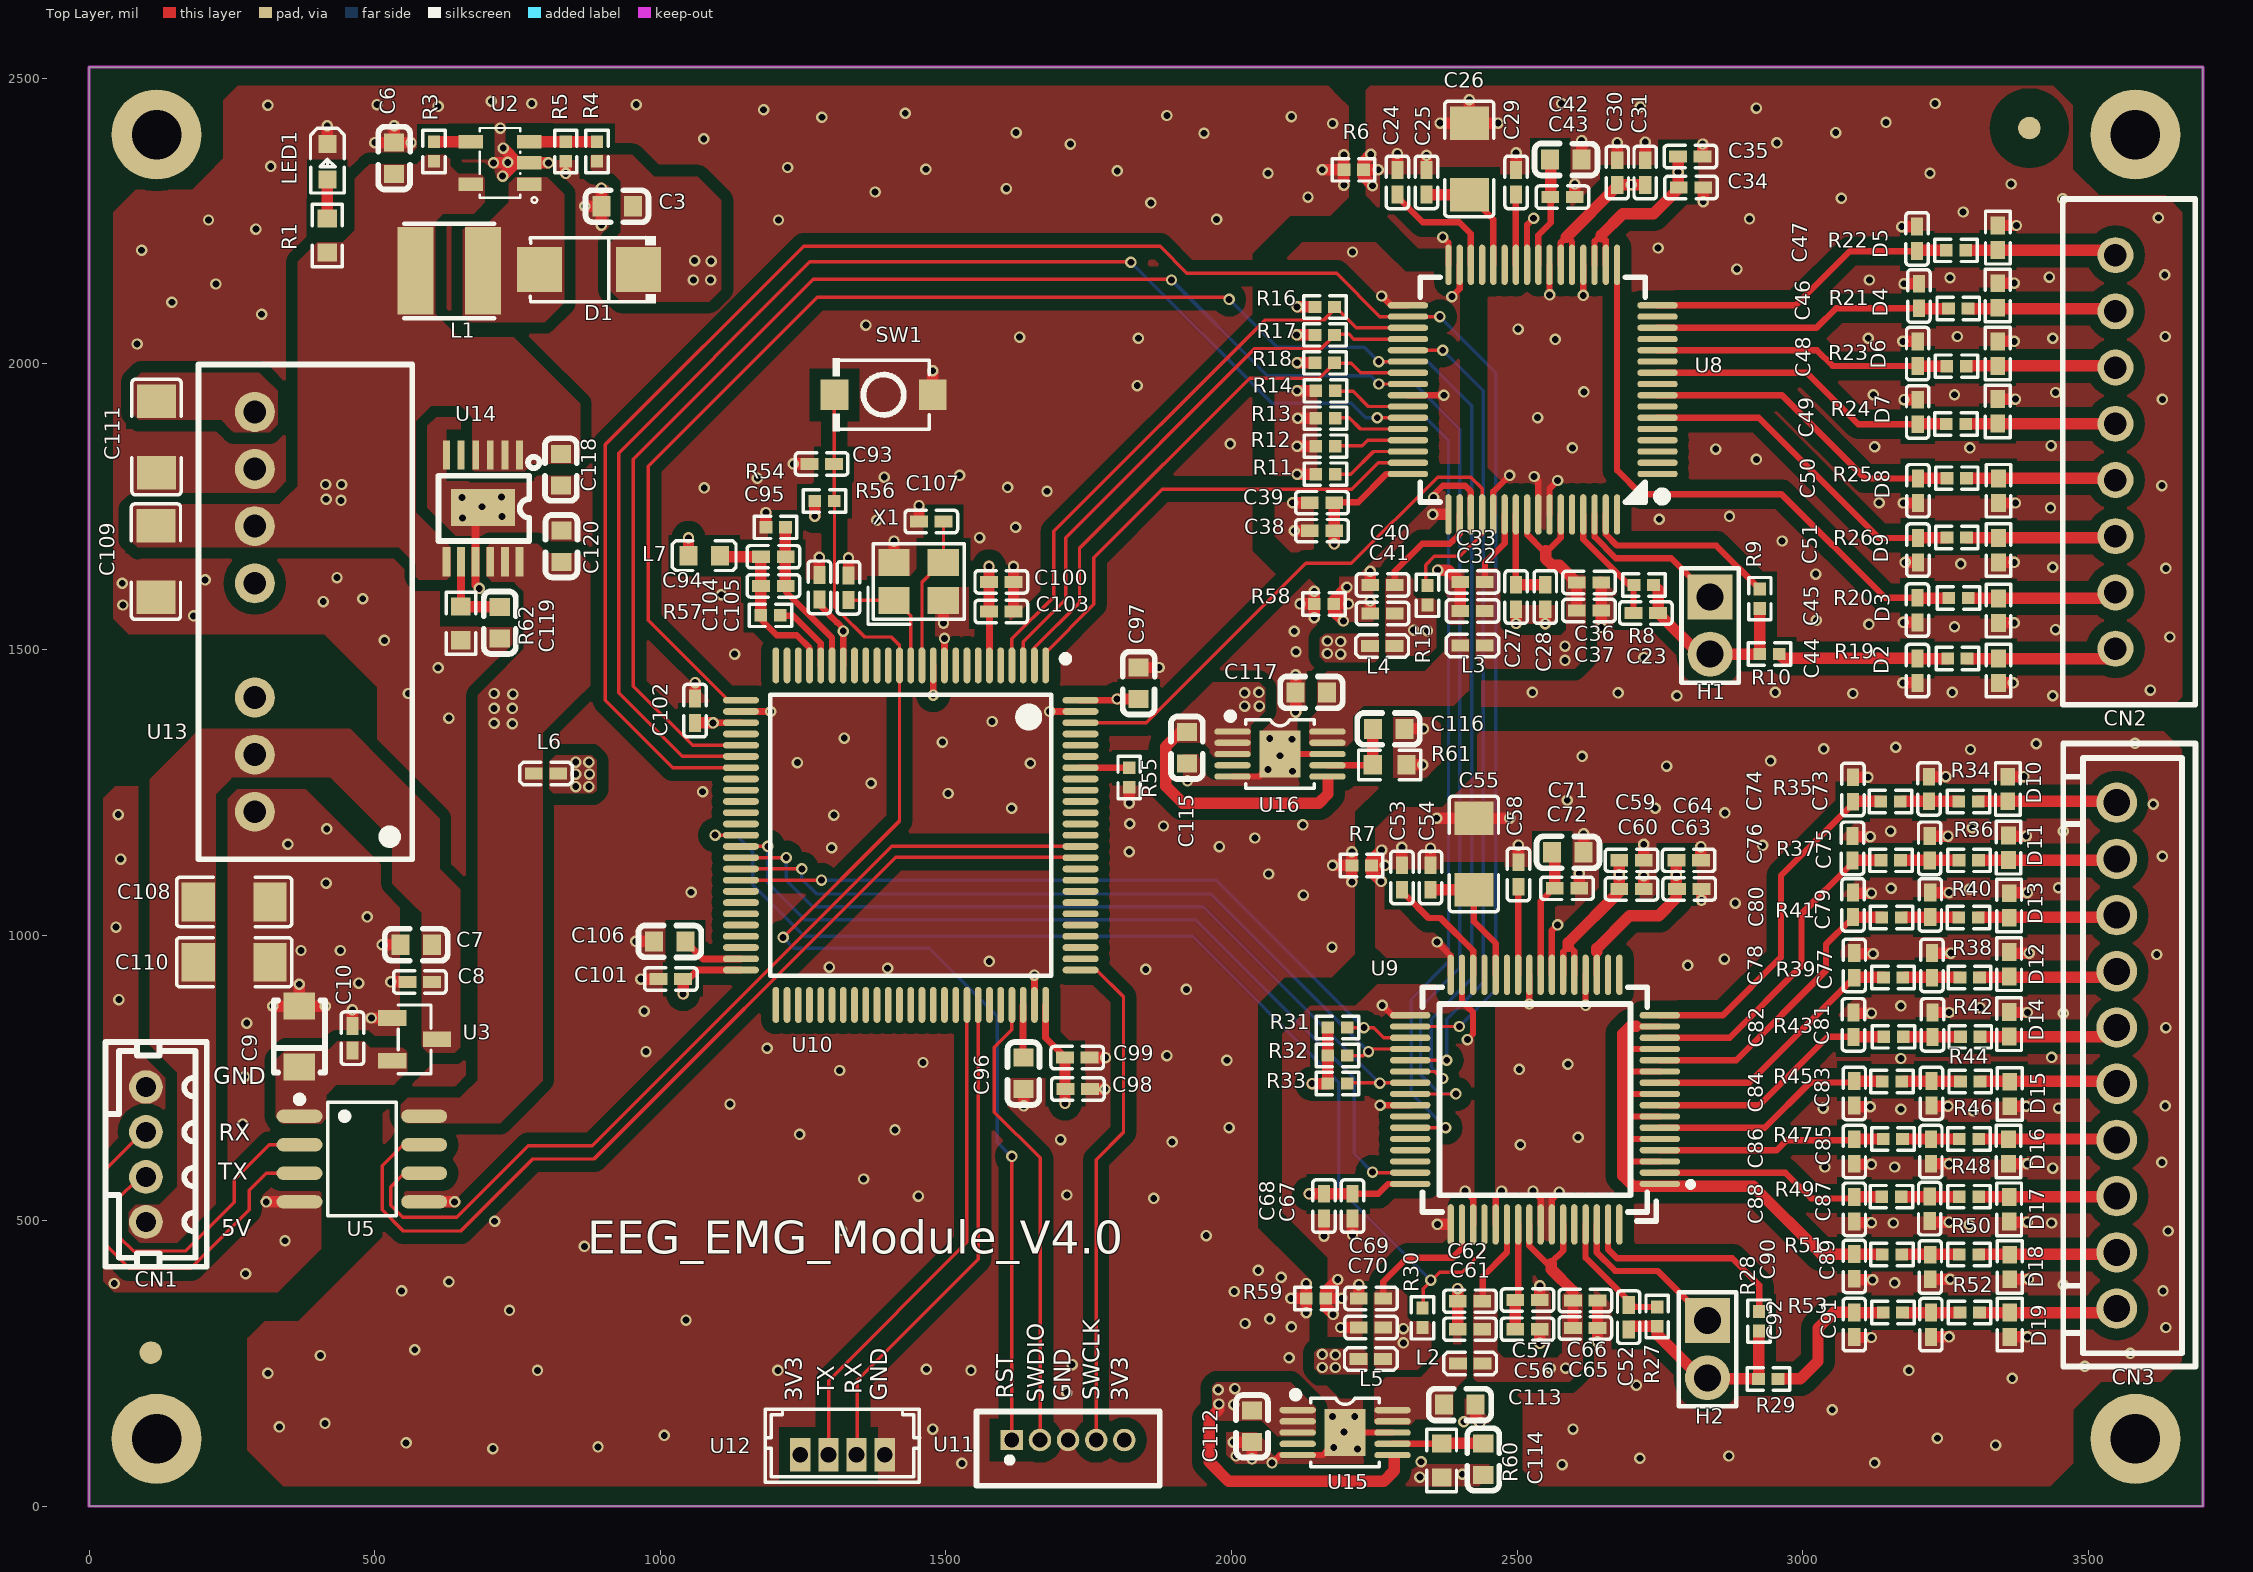
[diagram p0: Top Layer view]
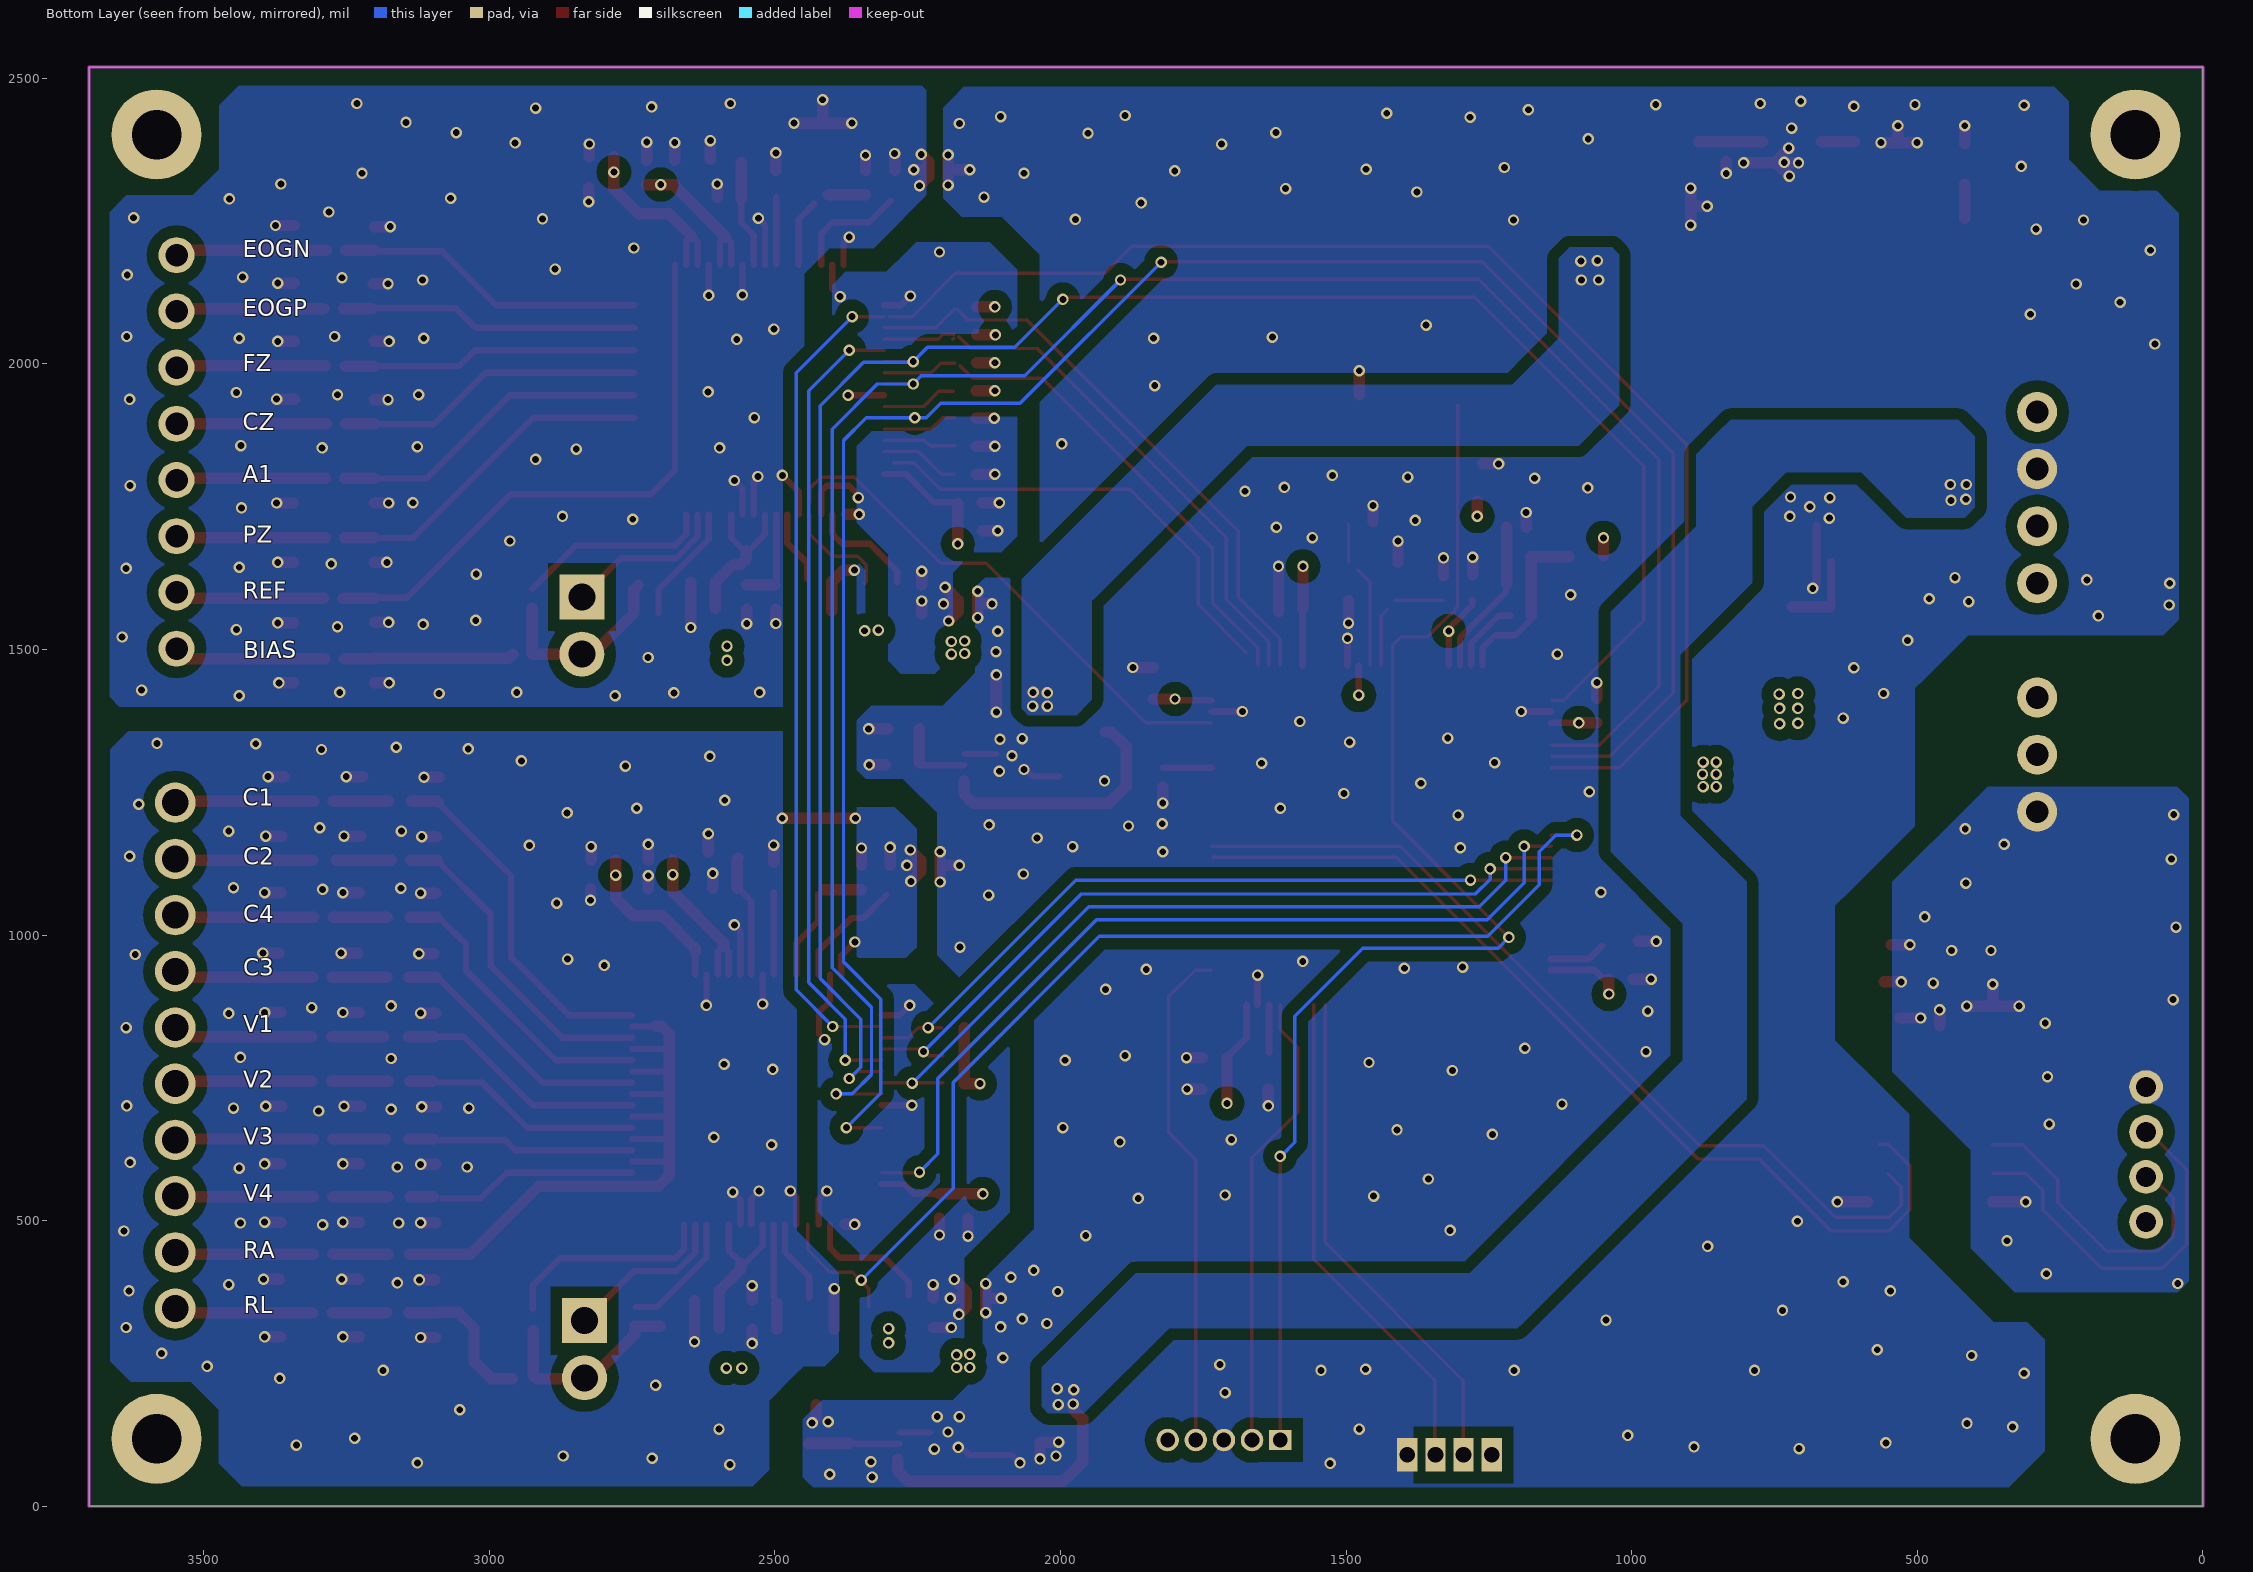
[diagram p1: Bottom Layer view, seen from below]
# Altium PCB MISC86293.PcbDoc (part 1 of 4)
Units mil, origin at the board's own origin, x right, y up, seen from the top; angles counter-clockwise.
Board outline 3700.79 x 2519.68 mil, 4 copper layers (Top Layer, GND, POWER, Bottom Layer); 211 components, 128 nets, 717 pads, 581 vias.

## Layer stack, top to bottom (the 12.6 mil dielectric is the usual default, probably not edited)
Top Layer: signal copper 1.4
Dielectric: core 12.6, FR-4, Dk 4.8
GND: plane copper 1.4, net (Multiple Nets)
Dielectric: prepreg 12.6, FR-4, Dk 4.8
POWER: plane copper 1.4, net (Multiple Nets)
Dielectric: core 12.6, FR-4, Dk 4.8
Bottom Layer: signal copper 1.4

## Board outline
0,0 0,2519.68 3700.79,2519.68 3700.79,0

## Design rules (kind name [scope] priority, off if disabled: settings)
Clearance Clearance_2 [HASPAD('FREE-MARK')] p1: gap=50
Clearance Clearance_1 [inpolygon] p2: gap=6
Clearance [All] p3: gap=6
HoleSize [All] p1: absolutevalues=TRUE maxlimit=500 minlimit=1 maxpercent=80.000 minpercent=20.000
HoleToHoleClearance [All] p1: gap=0 allowstackedmicrovias=TRUE
MinimumSolderMaskSliver [All] p1: minsoldermaskwidth=0
PlaneClearance [All] p1: clearance=6
PlaneConnect [All] p1: planeconnectstyle=Direct reliefexpansion=20 reliefentries=4 reliefconductorwidth=10 reliefairgap=10
PolygonConnect [All] p1: connectstyle=Direct reliefconductorwidth=10 reliefentries=4 polygonreliefangle="90 Angle"
RoutingVias [All] p1: holewidth=12 width=20 viastyle="Through Hole" minholewidth=12 minwidth=20 maxholewidth=12 maxwidth=20
SilkToSilkClearance [All] p1: silktosilkclearance=0
SilkscreenOverComponentPads [All] p1: minsilkscreentomaskgap=0
SolderMaskExpansion [All] p1: expansion=4
Width [All] p1: maxlimit=40 minlimit=6 preferedwidth=6 minimp=50.000000 maximp=50.000000 favimp=50.000000
21 further rules are at their usual default settings.

## Classes and differential pairs
component class 电源: C3 C6 C7 C8 C9 C10 C108 C109 C110 C111 C112 C113 C114 C115 C116 C117 C118 C119 C120 CN1 D1 L1 L2 L3 L4 L5 L6 LED1 R1 R3 R4 R5 R6 R7 R58 R59 R60 R61 R62 U2 U3 U5 U13 U14 U15 U16
component class STM32: C93 C94 C95 C96 C97 C98 C99 C100 C101 C102 C103 C104 C105 C106 C107 L7 R54 R55 R56 R57 SW1 U10 U11 U12 X1
component class EMG_ADS1298_引脚滤波: C73 C74 C75 C76 C77 C78 C79 C80 C81 C82 C83 C84 C85 C86 C87 C88 C89 C90 C91 C92 CN3 D10 D11 D12 D13 D14 D15 D16 D17 D18 D19 R34 R35 R36 R37 R38 R39 R40 R41 R42 R43 R44 R45 R46 R47 R48 R49 R50 R51 R52 R53
component class EMG_ADS1298_电源部分: C59 C60 C61 C62 C63 C64 C65 C66 C67 C68 C69 C70 C71 C72
component class EMG_ADS1298_功能模块: C52 C53 C54 C55 C56 C57 C58 H2 R27 R28 R29 R30 R31 R32 R33 U9
component class EEG_ADS1299_引脚滤波: C44 C45 C46 C47 C48 C49 C50 C51 CN2 D2 D3 D4 D5 D6 D7 D8 D9 R19 R20 R21 R22 R23 R24 R25 R26
component class EEG_ADS1299_电源部分: C30 C31 C32 C33 C34 C35 C36 C37 C38 C39 C40 C41 C42 C43
component class EEG_ADS1299_功能模块: C23 C24 C25 C26 C27 C28 C29 H1 R8 R9 R10 R11 R12 R13 R14 R15 R16 R17 R18 U8

## Components (designator, comment, footprint, x,y, rotation, side; value= is the part's Value field where it differs from the comment)
C3 "10uF" C0603#1 924.48,2276 r0 top
C6 "10uF" C0603#1 534,2360 r270 top
C7 "10uF" C0603#1 573,983 r0 top
C8 "1uF" C0402 579,918 r0 top
C9 "22uF" CAP-SMD_L3.2-W1.6 368,822.52 r90 top
C10 "1uF" C0402 461,819.52 r270 top
C23 "10nF" C0402 2725.48,1564 r180 top
C24 "1uF" C0402 2290.48,2318 r90 top
C25 "1uF" C0402 2341.48,2318 r270 top
C26 "100uF" C1206 2416.48,2359 r270 top
C27 "1uF" C0402 2498.48,1592 r90 top
C28 "100nF" C0402 2549.48,1592 r90 top
C29 "1uF" C0402 2498.48,2318 r90 top
C30 "1uF" C0402 2675.48,2335 r270 top
C31 "100nF" C0402 2724.48,2335 r270 top
C32 "1uF" C0402 2422,1567.52 r180 top
C33 "100nF" C0402 2422,1618.52 r180 top
C34 "1uF" C0402 2804.48,2309 r180 top
C35 "100nF" C0402 2803.48,2363 r180 top
C36 "1uF" C0402 2626,1617.48 r180 top
C37 "100nF" C0402 2626,1568.48 r180 top
C38 "1uF" C0402 2158.48,1708 r180 top
C39 "100nF" C0402 2158.48,1757 r180 top
C40 "1uF" C0402 2264.48,1613 r0 top
C41 "100nF" C0402 2264.48,1563 r0 top
C42 "10uF" C0603#1 2585.48,2358 r180 top
C43 "100nF" C0402 2579.48,2292 r180 top
C44 "4.7nF" C0402 3200.96,1463 r90 top
C45 "4.7nF" C0402 3200.96,1569 r90 top
C46 "4.7nF" C0402 3203.48,2119 r270 top
C47 "4.7nF" C0402 3200.48,2219 r270 top
C48 "4.7nF" C0402 3201.48,2018 r270 top
C49 "4.7nF" C0402 3201.48,1916 r270 top
C50 "4.7nF" C0402 3201.96,1778 r90 top
C51 "4.7nF" C0402 3201.96,1674 r90 top
C52 "1.5nF" C0402 2695.48,331 r90 top
C53 "1uF" C0402 2298.48,1101 r90 top
C54 "1uF" C0402 2348.48,1101 r270 top
C55 "22uF" C1206 2424.48,1142 r270 top
C56 "1uF" C0402 2518.48,310 r180 top
C57 "100nF" C0402 2518.48,361 r180 top
C58 "1uF" C0402 2502.48,1106 r90 top
C59 "1uF" C0402 2700.48,1131 r180 top
C60 "100nF" C0402 2700.48,1081 r180 top
C61 "1uF" C0402 2417.48,310 r180 top
C62 "100nF" C0402 2417.48,359 r180 top
C63 "1uF" C0402 2801.48,1081 r180 top
C64 "100nF" C0402 2800.48,1131 r180 top
C65 "1uF" C0402 2619.48,312 r180 top
C66 "100nF" C0402 2619.48,360 r180 top
C67 "1uF" C0402 2212,525.52 r270 top
C68 "100nF" C0402 2162,525.52 r270 top
C69 "1uF" C0402 2244.48,364 r0 top
C70 "100nF" C0402 2244.48,313 r0 top
C71 "10uF" C0603#1 2589,1145 r180 top
C72 "100nF" C0402 2587.48,1082 r180 top
C73 "47pF" C0402 3221.48,1256 r270 top
C74 "47pF" C0402 3088,1255 r270 top
C75 "47pF" C0402 3222.48,1152 r270 top
C76 "47pF" C0402 3087.48,1152 r270 top
C77 "47pF" C0402 3226.48,947 r270 top
C78 "47pF" C0402 3090.48,947 r270 top
C79 "47pF" C0402 3223.48,1053 r270 top
C80 "47pF" C0402 3088.48,1053 r270 top
C81 "47pF" C0402 3227.48,843 r270 top
C82 "47pF" C0402 3089,843 r270 top
C83 "47pF" C0402 3225.48,723 r90 top
C84 "47pF" C0402 3090.48,723 r90 top
C85 "47pF" C0402 3224.48,621 r90 top
C86 "47pF" C0402 3090.48,621 r90 top
C87 "47pF" C0402 3222.48,521 r90 top
C88 "47pF" C0402 3090.48,520 r90 top
C89 "47pF" C0402 3223.48,419 r90 top
C90 "47pF" C0402 3090.48,420 r90 top
C91 "47pF" C0402 3224.48,318 r90 top
C92 "47pF" C0402 3090.48,318 r90 top
C93 "100nF" C0402 1282.48,1825 r0 top
C94 "100nF" C0402 1198,1611.52 r180 top
C95 "1uF" C0402 1198,1662.52 r180 top
C96 "2.2uF" C0603#1 1636,758 r90 top
C97 "10uF" C0603#1 1837.48,1441 r270 top
C98 "100nF" C0402 1731,730.48 r180 top
C99 "100nF" C0402 1730,785.48 r180 top
C100 "100nF" C0402 1597,1618.52 r180 top
C101 "100nF" C0402 1018.48,923 r0 top
C102 "100nF" C0402 1061,1393 r270 top
C103 "100nF" C0402 1597,1566.52 r180 top
C104 "100nF" C0402 1278.48,1609 r270 top
C105 "12pF" C0402 1329.48,1608 r270 top
C106 "2.2uF" C0603#1 1016.48,989 r180 top
C107 "12pF" C0402 1474.48,1724 r0 top
C108 "100uF" C1206 254,1058 r0 top
C109 "100uF" C1206 117,1654 r270 top
C110 "47uF" C1206 254,952.52 r0 top
C111 "22uF" C1206 118,1872 r270 top
C112 "4.7uF" C0603#2 2036,140 r90 top
C113 "4.7uF" C0603#2 2400,178 r0 top
C114 "470nF" C0603#2 2441,82 r90 top
C115 "4.7uF" C0603#2 1922,1328 r90 top
C116 "470nF" C0603#2 2275,1361 r180 top
C117 "4.7uF" C0603#2 2140,1425 r180 top
C118 "4.7uF" C0603#2 826,1815 r90 top
C119 "470nF" C0603#2 719,1547 r90 top
C120 "10uF" C0603#2 827,1681 r270 top
CN1 "A2001WV-4P" CONN-TH_A2001WV-4P 99.48,616 r270 top
CN2 "WF-1A254A8P" CONN-TH_WF-1A254A8P 3547.78,1846 r270 top
CN3 "A2501WV-10P" CONN-TH_A2501WV-10P 3550,789 r270 top
D1 "B340LA-13-F" SMA_L4.3-W2.6-LS5.2-RD 875,2165 r180 top
D2 "TPD1E10B06DPYR-TP" X1-DFN1006-2_L1.0-W0.6-BI 3342.96,1463 r90 top
D3 "TPD1E10B06DPYR-TP" X1-DFN1006-2_L1.0-W0.6-BI 3342.96,1568 r90 top
D4 "TPD1E10B06DPYR-TP" X1-DFN1006-2_L1.0-W0.6-BI 3341.48,2120 r270 top
D5 "TPD1E10B06DPYR-TP" X1-DFN1006-2_L1.0-W0.6-BI 3342,2221 r270 top
D6 "TPD1E10B06DPYR-TP" X1-DFN1006-2_L1.0-W0.6-BI 3341.48,2018 r270 top
D7 "TPD1E10B06DPYR-TP" X1-DFN1006-2_L1.0-W0.6-BI 3341.48,1917 r270 top
D8 "TPD1E10B06DPYR-TP" X1-DFN1006-2_L1.0-W0.6-BI 3342.96,1778 r90 top
D9 "TPD1E10B06DPYR-TP" X1-DFN1006-2_L1.0-W0.6-BI 3342.96,1674 r90 top
D10 "TPD1E10B06DPYR-TP" X1-DFN1006-2_L1.0-W0.6-BI 3359.48,1256 r270 top
D11 "TPD1E10B06DPYR-TP" X1-DFN1006-2_L1.0-W0.6-BI 3360.48,1153 r270 top
D12 "TPD1E10B06DPYR-TP" X1-DFN1006-2_L1.0-W0.6-BI 3361.48,949 r270 top
D13 "TPD1E10B06DPYR-TP" X1-DFN1006-2_L1.0-W0.6-BI 3361.48,1052 r270 top
D14 "TPD1E10B06DPYR-TP" X1-DFN1006-2_L1.0-W0.6-BI 3361.48,844 r270 top
D15 "TPD1E10B06DPYR-TP" X1-DFN1006-2_L1.0-W0.6-BI 3362.48,722 r90 top
D16 "TPD1E10B06DPYR-TP" X1-DFN1006-2_L1.0-W0.6-BI 3360.48,621 r90 top
D17 "TPD1E10B06DPYR-TP" X1-DFN1006-2_L1.0-W0.6-BI 3361.48,520 r90 top
D18 "TPD1E10B06DPYR-TP" X1-DFN1006-2_L1.0-W0.6-BI 3362.48,419 r90 top
D19 "TPD1E10B06DPYR-TP" X1-DFN1006-2_L1.0-W0.6-BI 3362.48,318 r90 top
H1 "PZ254V-11-02P-YL" HDR-TH_2P-P2.54-V-M 2838,1542 r270 top
H2 "PZ254V-11-02P-YL" HDR-TH_2P-P2.54-V-M 2833.48,275 r270 top
L1 "4.7uH" IND-SMD_L4.0-W4.0_FNR40XXS 630.48,2163 r180 top
L2 "BLM15PD121SN1D" L0402 2418,250 r0 top
L3 "BLM15PD121SN1D" L0402 2422,1507 r0 top
L4 "BLM15PD121SN1D" L0402 2264,1506 r0 top
L5 "BLM15PD121SN1D" L0402 2244,258 r0 top
L6 "BLM15PD121SN1D" L0402 800,1283 r0 top
L7 "GZ1608D601TF" L0603 1077,1664 r0 top
LED1 "KT-0603R" LED0603-RD 417,2354 r270 top
R1 "" R0603 417,2225 r90 top
R3 "" R0402 604,2372 r270 top
R4 "" R0402 889.48,2372 r270 top
R5 "" R0402 834.48,2372 r90 top
R6 "" R0402 2214,2340 r180 top
R7 "" R0402 2228,1122 r180 top
R8 "" R0402 2722,1613 r0 top
R9 "" R0402 2925,1589 r270 top
R10 "" R0402 2942,1492 r0 top
R11 "" R0402 2164.48,1807 r180 top
R12 "" R0402 2164.48,1856 r180 top
R13 "" R0402 2164.48,1905 r180 top
R14 "" R0402 2164.48,1953 r180 top
R15 "" R0402 2343.48,1595 r270 top
R16 "" R0402 2163.48,2100 r180 top
R17 "" R0402 2163.48,2051 r180 top
R18 "" R0402 2163.48,2002 r180 top
R19 "" R0402 3270.96,1484 r180 top
R20 "" R0402 3272.96,1590 r180 top
R21 "" R0402 3272.48,2097 r180 top
R22 "" R0402 3268.48,2199 r180 top
R23 "" R0402 3269.48,1996 r180 top
R24 "" R0402 3268.48,1895 r180 top
R25 "" R0402 3269.96,1800 r180 top
R26 "" R0402 3269.96,1696 r180 top
R27 "" R0402 2745.48,332 r270 top
R28 "" R0402 2923.48,324 r270 top
R29 "" R0402 2940,223 r0 top
R30 "" R0402 2334.48,330 r270 top
R31 "" R0402 2185.48,838 r180 top
R32 "" R0402 2185.48,789 r180 top
R33 "" R0402 2185.48,740 r180 top
R34 "" R0402 3290.48,1234 r180 top
R35 "" R0402 3154,1234 r180 top
R36 "" R0402 3291,1131 r180 top
R37 "" R0402 3154.48,1131 r180 top
R38 "" R0402 3292.48,926 r180 top
R39 "" R0402 3158.48,926 r180 top
R40 "" R0402 3290.48,1031 r180 top
R41 "" R0402 3155.48,1031 r180 top
R42 "" R0402 3293.48,822 r180 top
R43 "" R0402 3159,822 r180 top
R44 "" R0402 3293.48,744 r180 top
R45 "" R0402 3156.48,744 r180 top
R46 "" R0402 3291.48,643 r180 top
R47 "" R0402 3158,643 r180 top
R48 "" R0402 3291.48,542 r180 top
R49 "" R0402 3155.48,542 r180 top
R50 "" R0402 3291.48,441 r180 top
R51 "" R0402 3156.48,441 r180 top
R52 "" R0402 3292.48,339 r180 top
R53 "" R0402 3158,339 r180 top
R54 "" R0402 1202,1714 r0 top
R55 "" R0402 1821,1276 r270 top
R56 "" R0402 1287.48,1760 r180 top
R57 "" R0402 1193,1560 r0 top
R58 "" R0402 2162,1580 r180 top
R59 "" R0402 2148,364 r180 top
R60 "" R0603 2368,80 r90 top
R61 "" R0603 2277,1298 r0 top
R62 "" R0603 651,1546 r90 top
SW1 "TS-1088-AR02016" SW-SMD_L3.9-W3.0-P4.45 1391,1946 r180 top
U2 "MT3540" SOT-23-5_L3.0-W1.7-P0.95-LS2.8-BR 719.48,2352 r0 top
U3 "LN6206P332MR-G" SOT-23-3_L2.9-W1.3-P1.90-LS2.4-BR 570,817.52 r180 top
U5 "" SOIC-8_L4.9-W3.9-P1.27-LS6.0-BL 477.48,608 r270 top
U8 "ADS1299IPAGR" TQFP-64_L10.0-W10.0-P0.50-LS12.0-TL 2527.48,1955 r180 top
U9 "ADS1298IPAGR" TQFP-64_L10.0-W10.0-P0.50-LS12.0-BL 2531.48,712 r90 top
U10 "STM32F407VGT6" LQFP-100_L14.0-W14.0-P0.50-LS16.0-BL 1438.48,1175 r180 top
U11 "WAFER-MX1.25-5PZZ" CONN-TH_5P-P1.25_XUNPU_WAFER-MX1.25-5PZZ 1714,116 r0 top
U12 "WAFER-MX1.25-4PZZ" CONN-TH_4P-P1.25_WAFER-MX1.25-4PZZ 1319,90 r180 top
U13 "WRB0505S-3WR2" PWRM-TH_WRA0512S-3WR2 290,1566 r90 top
U14 "LT3045EMSE#TRPBF" MSOP-12_L4.0-W3.0-P0.65-LS4.9-BL-EP 689.52,1747 r180 top
U15 "LT3042EMSE#TRPBF" MSOP-10_L3.0-W3.0-P0.50-LS5.0-BL-EP 2199,129 r270 top
U16 "LT3042EMSE#TRPBF" MSOP-10_L3.0-W3.0-P0.50-LS5.0-BL-EP 2085,1317 r270 top
X1 "8MHz" CRYSTAL-SMD_4P-L3.2-W2.5-BL 1452.48,1619 r0 top

## Footprints (in the part's own frame and the unit in brackets; to place one, negate y for a bottom-side part, rotate by r counter-clockwise, add the part's x,y. Pads: shape width x height; smd on the part's side, far side on the other; paste and mask are expansions set on the pad)
C0402 [mm]
  rect 0.79x0.54 smd paste-100 mask+0.051: 1(-0.545,0) 2(0.545,0)
  silkscreen extent -1.17,-0.5 1.17,0.5
C0603#1 [mm]
  rect 0.8x0.9 smd: 1(-0.7,0) 2(0.7,0)
  silkscreen extent -1.41,-0.71 1.39,0.72
C0603#2 [mm]
  rect 0.8x0.9 smd paste+0.051 mask+0: 1(-0.7,0) 2(0.7,0)
  silkscreen extent -1.39,-0.71 1.39,0.71
C1206 [mm]
  rect 1.485x1.728 smd paste-100 mask+0.051: 1(-1.593,0) 2(1.593,0)
  silkscreen extent -2.56,-1.09 2.56,1.09